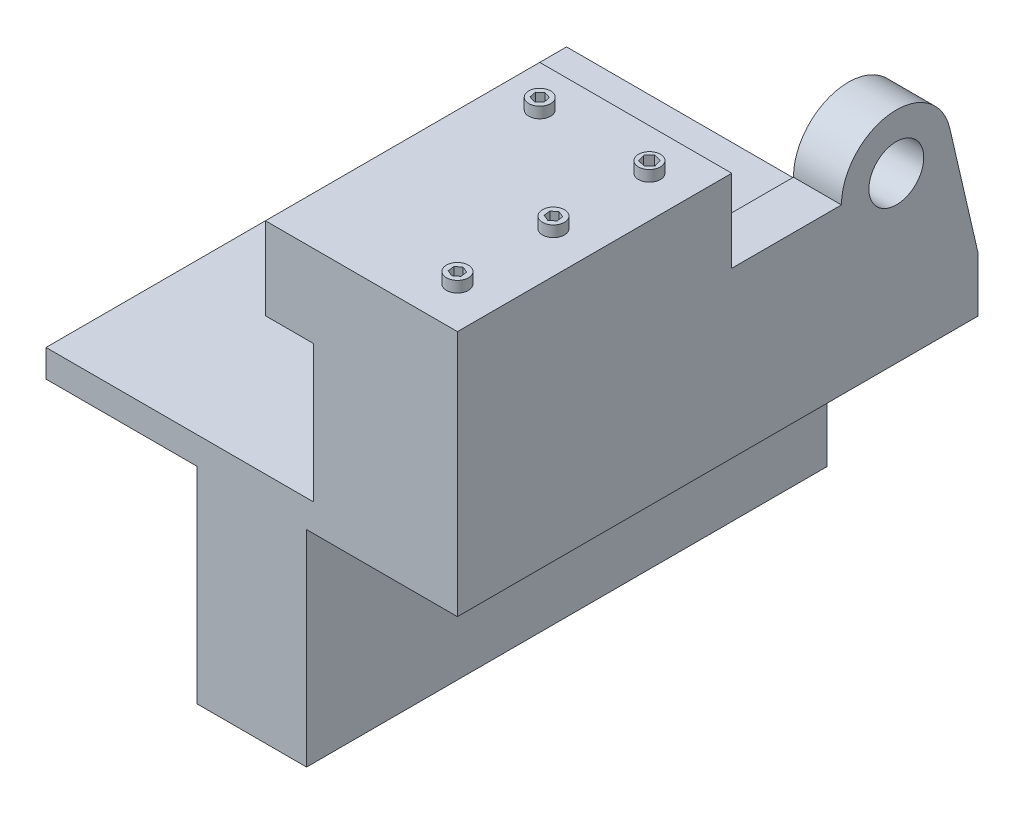
SolidWorks part; units mm, degrees
ref_plane "Front Plane" through (0, 0, 0) normal (0, 0, 1) x (1, 0, 0)
ref_plane "Top Plane" through (0, 0, 0) normal (0, 1, 0) x (1, 0, 0)
ref_plane "Right Plane" through (0, 0, 0) normal (1, 0, 0) x (0, 0, -1)
other "Configuration Table"
sketch "Sketch1" plane through (0, 0, 0) normal (0, 1, 0) x (1, 0, 0)
  line L1 (-35, 50) -> (35, 50)
  line L2 (-35, 50) -> (-35, -50)
  line L3 (-35, -50) -> (35, -50)
  line L4 (35, 50) -> (35, -50)
  line L5 (-35, 50) -> (35, -50) construction
  line L6 (-35, -50) -> (35, 50) construction
  point P0 (0, 0)
  dimension "D1" = 70
  dimension "D2" = 100
extrude "Boss-Extrude1" add sketch "Sketch1" along normal blind 30
sketch "Sketch2" plane through (0, 30, 0) normal (0, 1, 0) x (1, 0, 0)
  line L0 (20, 50) -> (20, -35) construction
  line L1 (35, 50) -> (-35, 50) construction
  line L2 (20, -35) -> (-35, -35) construction
  line L3 (-35, 50) -> (-35, -50) construction
  line L4 (35, -50) -> (35, 50) construction
  line L5 (-35, -50) -> (35, -50) construction
  line L7 (21.9131, 33.5347) -> (22.2255, 35.9241)
  line L8 (22.2255, 35.9241) -> (20.3125, 37.3894)
  line L9 (20.3125, 37.3894) -> (18.0869, 36.4653)
  line L10 (18.0869, 36.4653) -> (17.7745, 34.0759)
  line L11 (17.7745, 34.0759) -> (19.6875, 32.6106)
  line L12 (19.6875, 32.6106) -> (21.9131, 33.5347)
  line L13 (21.9131, -1.4702) -> (22.2298, 0.9217)
  line L14 (22.2298, 0.9217) -> (20.3167, 2.3919)
  line L15 (20.3167, 2.3919) -> (18.0869, 1.4702)
  line L16 (18.0869, 1.4702) -> (17.7702, -0.9217)
  line L17 (17.7702, -0.9217) -> (19.6833, -2.3919)
  line L18 (19.6833, -2.3919) -> (21.9131, -1.4702)
  line L19 (21.9131, -37.0352) -> (22.719, -34.3608)
  line L20 (22.719, -34.3608) -> (20.806, -32.3257)
  line L21 (20.806, -32.3257) -> (18.0869, -32.9648)
  line L22 (18.0869, -32.9648) -> (17.281, -35.6392)
  line L23 (17.281, -35.6392) -> (19.194, -37.6743)
  line L24 (19.194, -37.6743) -> (21.9131, -37.0352)
  line L25 (-18.1325, -36.6568) -> (-17.6315, -34.2111)
  line L26 (-17.6315, -34.2111) -> (-19.4989, -32.5543)
  line L27 (-19.4989, -32.5543) -> (-21.8675, -33.3432)
  line L28 (-21.8675, -33.3432) -> (-22.3685, -35.7889)
  line L29 (-22.3685, -35.7889) -> (-20.5011, -37.4457)
  line L30 (-20.5011, -37.4457) -> (-18.1325, -36.6568)
  circle A0 centre (-20, -35) radius 4
  circle A1 centre (20, -35) radius 4
  circle A2 centre (20, 0) radius 4
  circle A3 centre (20, 35) radius 4
  circle A4 centre (20, 35) radius 2.0869 construction
  circle A5 centre (20, 0) radius 2.0895 construction
  circle A6 centre (20, -35) radius 2.4189 construction
  circle A7 centre (-20, -35) radius 2.162 construction
  dimension "D3" = 8
  dimension "D4" = 8
  dimension "D5" = 8
  dimension "D6" = 8
  dimension "D1" = 15
  dimension "D2" = 15
  dimension "D7" = 15
  dimension "D8" = 35
  dimension "D9" = 35
extrude "Boss-Extrude2" add sketch "Sketch2" along normal blind 4
sketch "Sketch3" plane through (0, 0, 0) normal (0, -1, 0) x (1, 0, 0)
  line L0 (-35, 50) -> (35, 50) construction
  line L1 (17.5, -50) -> (-17.5, -50)
  line L2 (17.5, -50) -> (17.5, 50)
  line L3 (17.5, 50) -> (-17.5, 50)
  line L4 (-17.5, -50) -> (-17.5, 50)
  line L5 (17.5, -50) -> (-17.5, 50) construction
  line L6 (17.5, 50) -> (-17.5, -50) construction
  point P0 (0, 0)
  dimension "D1" = 35
extrude "Boss-Extrude3" add sketch "Sketch3" along normal blind 40
sketch "Sketch4" plane through (17.5, 0, 0) normal (1, 0, 0) x (0, 0, -1)
  line L0 (50, 0) -> (-50, 0) construction
  line L1 (-50, -40) -> (-139.7812, -40)
  line L2 (-139.7812, -40) -> (-129.4854, 4.5075)
  line L3 (-90, 0) -> (-50, 0)
  line L4 (-50, 0) -> (50, 0)
  line L5 (50, 0) -> (50, -40)
  line L6 (50, -40) -> (-50, -40)
  circle A0 centre (-110, 0) radius 10
  arc A1 (-90, 0) -> (-129.4854, 4.5075) centre (-110, 0) ccw
  dimension "D2" = 20
  dimension "D3" = 40
  dimension "D1" = 0
  dimension "D4" = 40
extrude "Boss-Extrude4" add sketch "Sketch4" along normal up to surface (17.5 mm away) up to face at (35, 15, 0)
sketch "Sketch5" plane through (0, -40, 0) normal (0, -1, 0) x (1, 0, 0)
  line L0 (17.5, 139.7812) -> (35, 139.7812)
  line L1 (35, 139.7812) -> (35, -50)
  line L2 (35, -50) -> (-17.5, -50)
  line L3 (-17.5, -50) -> (-17.5, 50)
  line L4 (-17.5, 50) -> (17.5, 50)
  line L5 (17.5, 50) -> (17.5, 139.7812)
extrude "Boss-Extrude5" add sketch "Sketch5" along normal blind 10
sketch "Sketch6" plane through (0, -50, 0) normal (0, -1, 0) x (1, 0, 0)
  line L0 (35, -50) -> (35, 139.7812) construction
  line L1 (35, -50) -> (-115, -50)
  line L2 (35, -50) -> (35, 139.7812)
  line L3 (35, 139.7812) -> (-115, 139.7812)
  line L4 (-115, -50) -> (-115, 139.7812)
  dimension "D1" = 150
extrude "Boss-Extrude6" add sketch "Sketch6" along normal blind 10
sketch "Sketch7" plane through (0, -60, 0) normal (0, -1, 0) x (1, 0, 0)
  line L0 (-115, 139.7812) -> (35, -50) construction
  line L1 (35, 139.7812) -> (-115, 139.7812) construction
  line L2 (-20, -50) -> (-60, -50)
  line L3 (-20, -50) -> (-20, 139.7812)
  line L4 (-20, 139.7812) -> (-60, 139.7812)
  line L5 (-60, -50) -> (-60, 139.7812)
  line L6 (-20, -50) -> (-60, 139.7812) construction
  line L7 (-20, 139.7812) -> (-60, -50) construction
  line L8 (35, -50) -> (35, 139.7812) construction
  point P4 (-40, 44.8906)
  dimension "D1" = 55
extrude "Boss-Extrude7" add sketch "Sketch7" along normal blind 75
ref_plane "Plane1" through (40.5, 0, 0) normal (1, 0, 0) x (0, 0, -1)
mirror "Mirror3" about plane through (17.5, -50, 139.7812) normal (0, 0, -1) of bodies 112
ref_plane "Plane2" through (0, 0, 139.7812) normal (0, 0, 1) x (1, 0, 0)
sketch "Sketch8" plane through (0, 0, 139.7812) normal (0, 0, 1) x (1, 0, 0)
  line L1 (-143.8581, 54.4321) -> (69.567, 54.4321)
  line L2 (-143.8581, 54.4321) -> (-143.8581, -147.136)
  line L3 (-143.8581, -147.136) -> (69.567, -147.136)
  line L4 (69.567, 54.4321) -> (69.567, -147.136)
extrude "Cut-Extrude1" cut sketch "Sketch8" against normal blind 210
